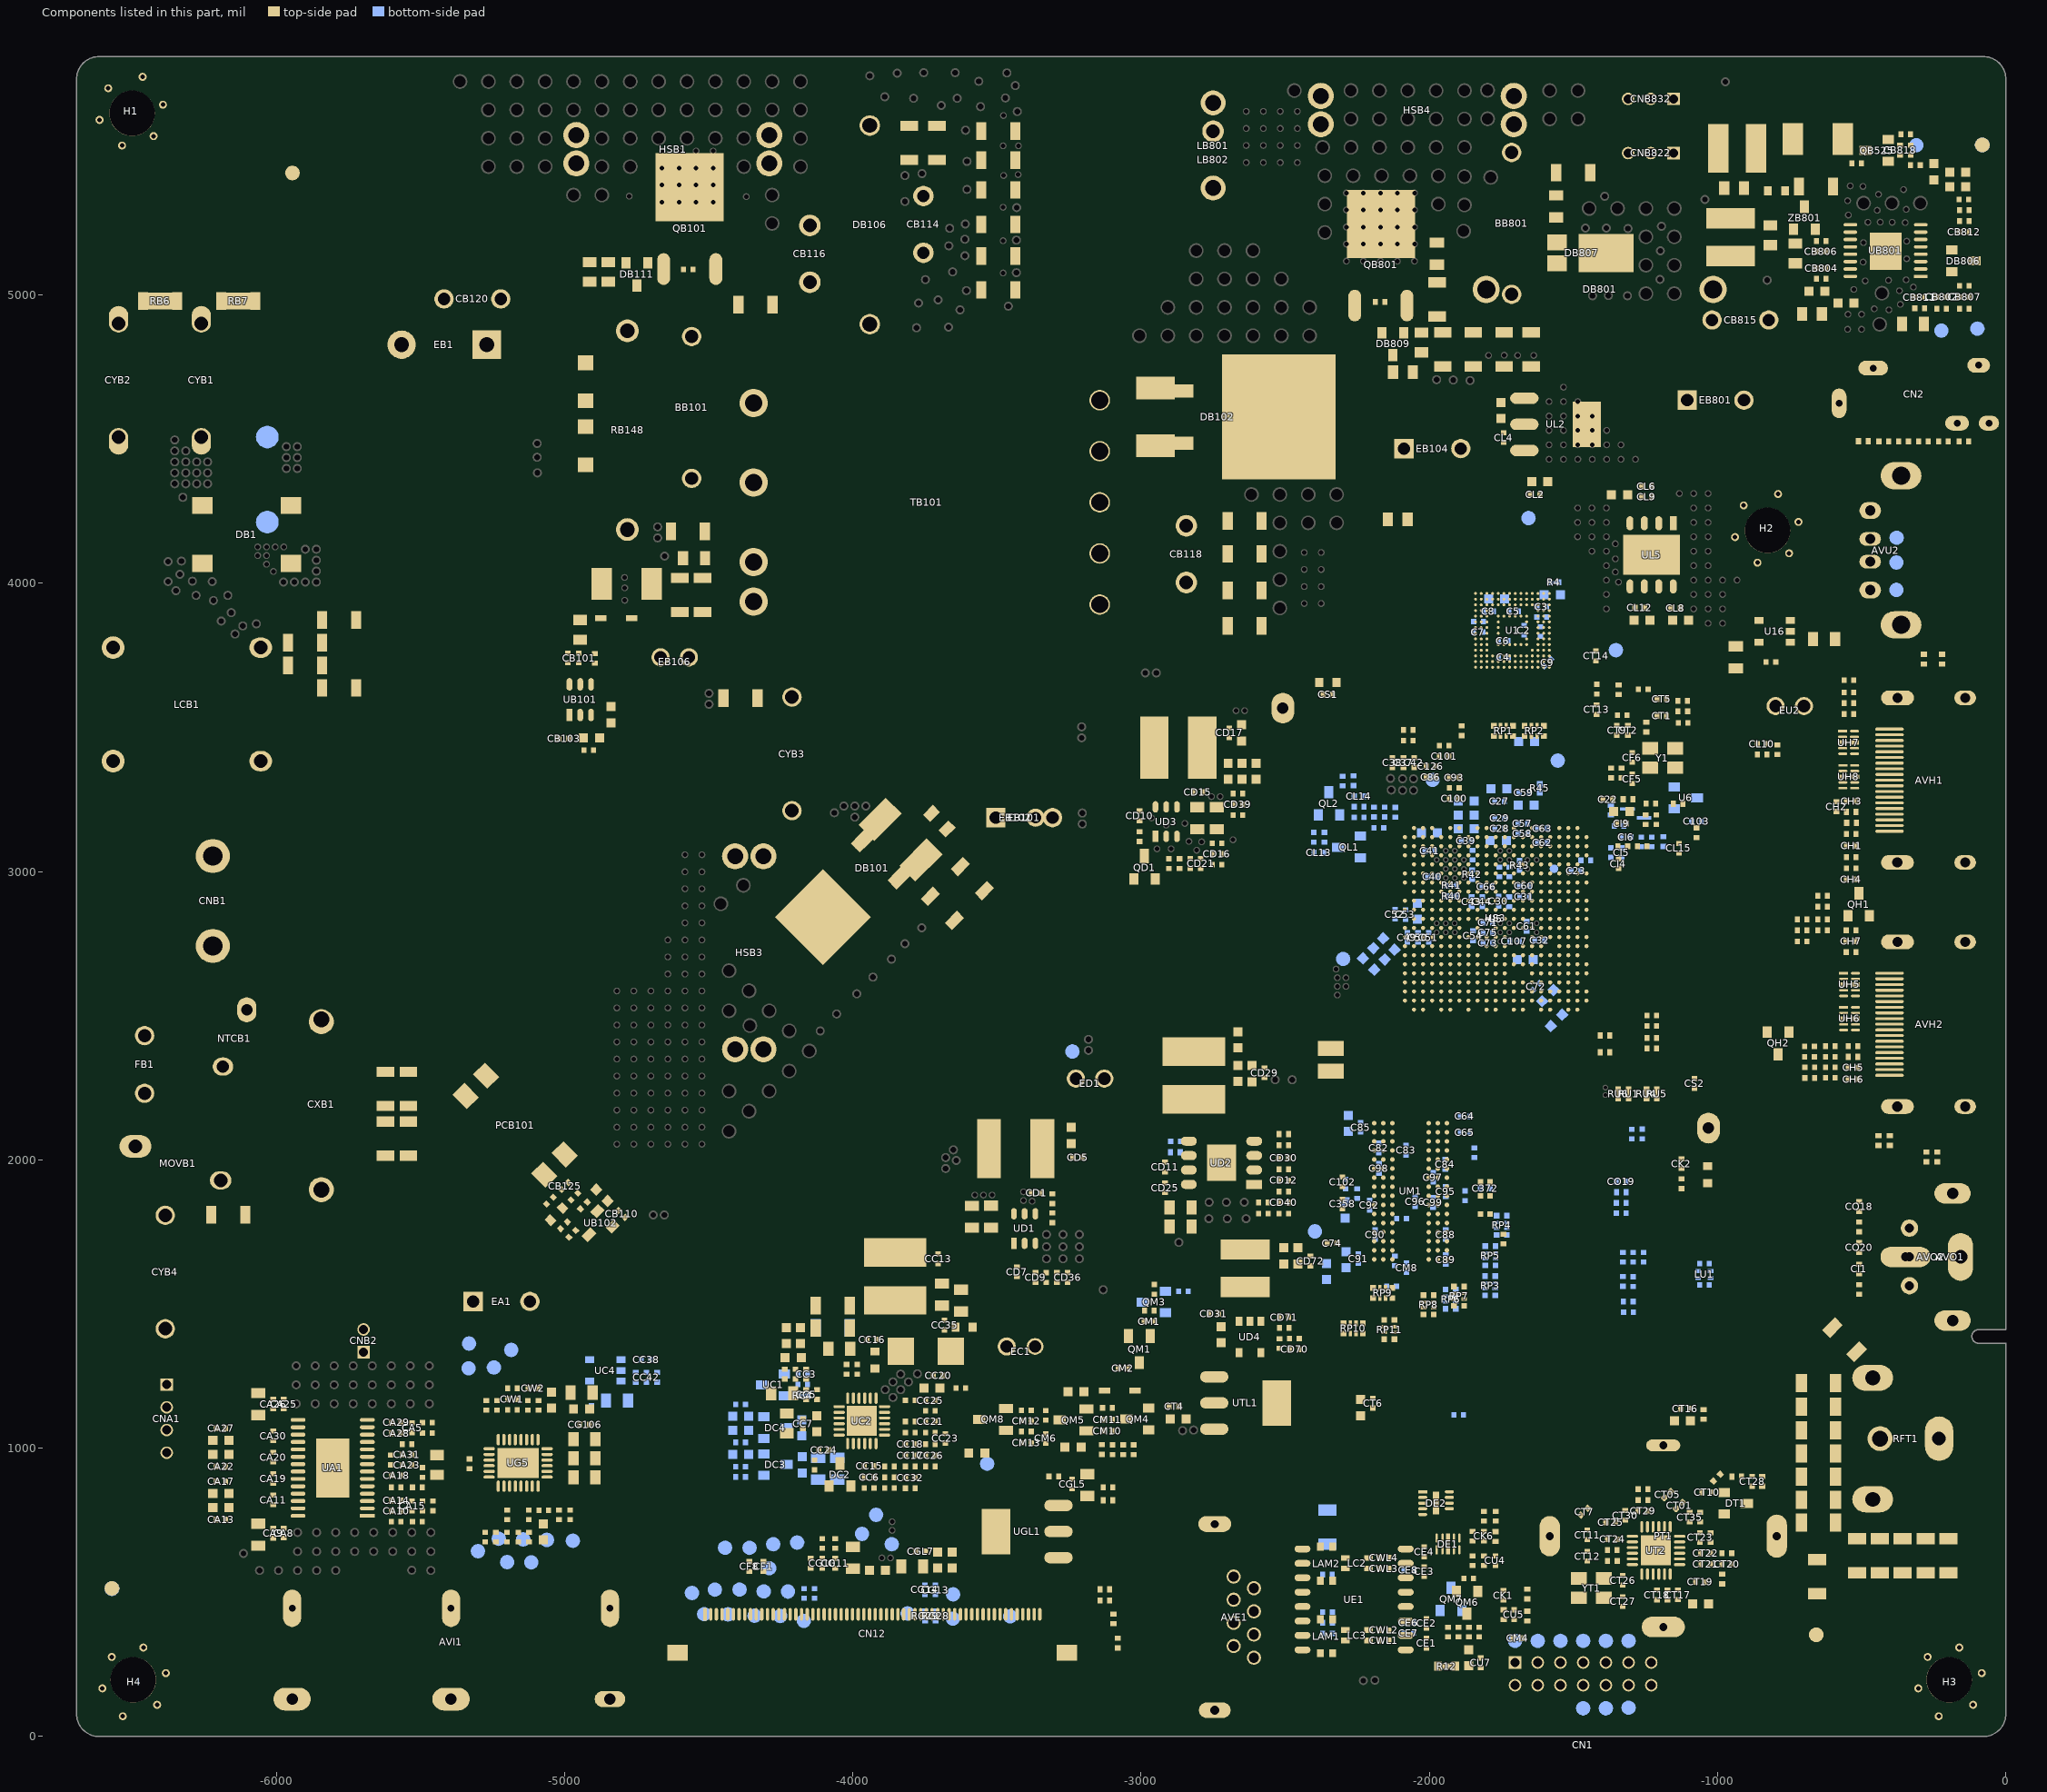
[diagram p0: the components of this part, seen from the top]
# Altium PCB MISC84395.PcbDoc (part 25 of 26)
Units mil, origin at the board's own origin, x right, y up, seen from the top; angles counter-clockwise.
Board outline 6692.91 x 5826.77 mil, 2 copper layers (TopLayer, BottomLayer), stack 61.855 mil thick; 951 components, 565 nets, 4374 pads, 1804 vias.
Unrouted connection lines stored in the file: 1.

## Keep-outs
KeepOutLayer:
  rectangle: 3183.8,-158.59 3314,-79.85
  pour cut-out: -6106,0 -6106,296 -6077,325 -4781.9,325 -4781.9,345 -6088,345 -6132,301 -6132,42 -6174,0
  pour cut-out: -2271,766 -2209,704 -2209,225 -2274,160 -2788,160 -2841,213 -2841,655 -2792,704 -2664.31,704 -2602.31,766
  lines w5: -172,0 -93.26,0 ; 0,118.11 0,590.55 ; 3734.7,-158.59 3734.7,-79.85 ; -6692.91,78.74 ccw(c-6614.17,78.74) -6614.17,0 -78.74,0 ccw(c-78.74,78.74) 0,78.74 0,1364.17 ; -6692.91,78.74 cw(c-6771.65,78.74) -6771.65,0 -13307.09,0 cw(c-13307.09,78.74) -13385.83,78.74 -13385.83,4415.35 -13291.34,4415.35 ccw(c-13291.34,4438.98) -13267.72,4438.98 ccw(c-13291.34,4438.98) -13291.34,4462.6 -13385.83,4462.6 -13385.83,5748.03 cw(c-13307.09,5748.03) -13307.09,5826.77 -6771.65,5826.77 cw(c-6771.65,5748.03) -6692.91,5748.03 ; -6692.91,78.74 -6692.91,5748.03 ; -6692.91,78.74 -6692.91,5748.03 ; -6692.91,5748.03 cw(c-6614.17,5748.03) -6614.17,5826.77 ; -6692.91,5748.03 cw(c-6614.17,5748.03) -6614.17,5826.77 ; -6692.91,5748.03 cw(c-6614.17,5748.03) -6614.17,5826.77 ; -6614.17,5826.77 -78.74,5826.77 ; -78.74,5826.77 cw(c-78.74,5748.03) 0,5748.03 ; -78.74,5826.77 cw(c-78.74,5748.03) 0,5748.03 ; 0,1364.17 -94.49,1364.17 cw(c-94.49,1387.8) -118.11,1387.8 cw(c-94.49,1387.8) -94.49,1411.42 0,1411.42 0,5748.03 ; 0,1364.17 0,1364.17 ; 3183.8,-158.59 3915.83,-158.59 3915.83,-79.85 3183.8,-79.85 3183.8,-158.59
  text "KeepOutLayer" at 3336.6,-137.63 h60
  text ".GKO" at 3758.41,-140.54 h60

## Other copper
TopLayer:
  drawing of 329 lines, arcs and shapes, not listed
  text "TopLayer" at 3349.85,461.03 h60
  text ".GTL" at 3759.34,456.74 h60
BottomLayer:
  drawing of 259 lines, arcs and shapes, not listed
  text ".GBL" at 3759.02,242.51 h60
  text "BottomLayer" at 3336.6,241.01 h60

## Silkscreen, mask and mechanical layers (free items; w line width, h text height)
TopOverlay:
  drawing of 503 lines, arcs and shapes, not listed
  text "LED DRIVER" at -1021.92,5754.78 h60
  text "2" at -7656.83,5661.77 h160 r180
  text "Solder Mask:" at 3048.92,5399.14 h60
  text "IPC SM-840" at 3461.42,5398.14 h60
  text "Silkscreen Color:" at 4227.42,5398.14 h60
  text "White" at 4706.42,5398.14 h60
  text "Units:" at 4227.42,5299.14 h60
  text "PTH Copper Thickness:" at 3048.92,5298.14 h60
  text ">20um" at 3722.42,5297.14 h60
  text "mm" at 4425.42,5297.64 h60
  text "Dielectric Constant Er@1GHz To 1MHz:" at 3048.58,5199.17 h60
  text "4.2 --- 4.6" at 4228.08,5199.67 h60
  text "Panel Size:" at 3046.92,5100.64 h60
  text "2L,2,170.00×148.00mm,FR4(TG130-CTI175),1OZ,Green,OSP,1.6mm" at 3352.08,5100.67 h60
  text "Silkscreen on PTH:" at 3047.42,4999.14 h60
  text "Primary Side Retained;" at 3565.42,4998.14 h60
  text "Secondary Side  Removed for Soldering" at 4227.42,4996.64 h60
  text "Special Requirements" at 3046.41,4908.46 h60
  text "If engineering questions are not answered within 2 hours, please call: PHONE_A" at 4933.08,4901.17 h60
  text "1. Lead-free HASL (HAL_LF, Lead Free Hot Air Leveling)" at 3637.3,4804.87 h60
  text "2. OSP (OSP, Organic Solderability Preservatives)" at 3637.3,4720.87 h60
  text "3. ENIG (ENIG, Electroless Nickel/Immersion Gold)" at 3635.8,4629.37 h60
  text "Plated Technics" at 3121.42,4594.64 h60
  text "4. ENIG + gold finger (ENIG_G/F, Electroless Nickel/Immersion Gold + Gold Finger)" at 3637.3,4548.87 h60
  text "5. Gold plating (Gold_plated, Gold-plated)" at 3638.3,4468.37 h60
  text "6. Gold plating + gold finger (Gold_Plated_G/F, Gold-plated + Gold Finger)" at 3638.8,4390.37 h60
  text "Impedance Control" at 3051.15,4161.78 h60
  text "Target Impedance" at 3847.98,4161.88 h60
  text "Layer(s)" at 5362.12,4161.96 h60
  text "Width & Clearance" at 4593.81,4161.65 h60
  text "75 +/- 10% Ohm" at 3870.18,4061.18 h60
  text "G/12/15.8/12/G mil" at 4551.23,4060.5 h60
  text "layer 1" at 5362.12,4060.62 h60
  text "Single End Impedance" at 3051.15,4014.96 h60
  text "[ Zo ]" at 3274.65,3877.71 h60
  text "G/5/7/5/7/5/G mil" at 4561.23,3669.5 h60
  text "100 +/- 10% Ohm" at 3857.18,3668.49 h60
  text "layer 1" at 5373.11,3666.71 h60
  text "Differential Impedance" at 3051.01,3613.38 h60
  text "[ Zo ]" at 3274.14,3490.05 h60
  text "( G: Ground )" at 3184.22,3382.55 h60
  text "90 +/- 10% Ohm" at 3883.23,3370.5 h60
  text "layer 1&2" at 5369.11,3369.71 h60
  text "G/5/11/5/11/5/G mil" at 4561.23,3367 h60
  text "Common Mode Impedance" at 3030.79,3160.87 h60
  text "[ Zc ]" at 3278.79,3079.87 h60
  text "Refer to Gerber documents GTP&GBP for Stencil aperture design" at 3945.84,2815.68 h60
  text "Stencil" at 3045.08,2718.67 h60
  text "TOP:New" at 3947,2714 h60
  text "BOTTOM:The Same As XXXXXXXXXXXXXXXX XXXXXX" at 3948,2618 h60
  text "Test jig" at 3043.17,2523.02 h60
  text "The Same As XXXXXXXXXXXXXXXX XXXXXX" at 3947.74,2520.12 h60
  text "Wave-soldering jig" at 3045.38,2424.78 h60
  text "The Same As XXXXXXXXXXXXXXXX XXXXXX" at 3951.74,2420.12 h60
  text "Solder paste" at 3943.36,2323 h60
  text "Production process" at 3043.86,2321.5 h60
  text "Note: depanel from the back side" at 4329,2318 h60
  text "This board is 340*148mm, overlength; please pay special attention in production." at 3943.08,2237.17 h60
  text "[Process and notes]" at 3224.08,2236.67 h60
  text "Special requirements" at 3044.86,2123.5 h60
  text "SMD components higher than 2mm on the wave-soldering side" at 3044.58,2022.17 h60
  text "Packaging notes" at 3044.24,1925.95 h60
  text "[Components prone to collision]" at 3285.58,1841.17 h60
  text "Footprint matching" at 3044.24,1725.95 h60
  text "CN1  CN2   AVE1" at 3941.73,1671 h60
  text "[New component footprint]" at 3271.58,1642.17 h60
  text "(Automated Testing Support)" at 3362.58,1527.67 h45
  text "Automatic test support" at 3044.08,1524.17 h60
  text "[Reserved suction cup and press bar positions]" at 3204.58,1439.67 h60
  text "12V" at -5556,1404 h50
  text "GND" at -5557,1318 h50
  text "PWR UPGRADE" at -6244,1312 h60
  text "Layer Stack Up Detail for" at 3185.18,1080.14 h100
  text ".Pcb_File_Name_No_Path" at 4246,1080.14 h100
  text "Layer" at 3349.54,932.41 h50
  text "Gerber" at 3721.26,932.41 h50
  text "Layer" at 4032.4,932.41 h50
  text "Layer" at 4668.64,932.41 h50
  text "Copper" at 5457.54,932.41 h50
  text "Dielectric" at 5769.32,932.41 h50
  text "Stack up" at 4668.64,881.53 h50
  text "Height" at 5769.32,881.53 h50
  text "Name" at 3349.54,880.03 h50
  text "Document" at 3721.26,880.03 h50
  text "Ordor" at 4032.4,880.03 h50
  text "Thickness" at 5457.54,880.03 h50
  text "SPEAKER" at -6666,837 h60
  text "TCON" at -4592,678 h60
  text "TopOverlay" at 3349.24,647.18 h60
  text ".GTO" at 3758.81,644.62 h60
  text "0.4mil" at 5766.64,559.59 h60
  text "1" at 4085.61,456.44 h60
  text "1.4mil" at 5470.6,456.38 h60
  text "2" at 4085.66,243.4 h60
  text "1.4mil" at 5468.89,242.39 h60
  text "1" at -5729,165 h160
  text "0.4mil" at 5769.31,147.71 h60
  text "KEY&IR&LED&EXT-WIFI" at -1082,47 h60
  text "Notes:" at 3021.11,-415.17 h80
  text "1. No Plated Through Hole  overlap each other should be combined ,Residues between them should be eliminated." at 3020.24,-503.08 h60
  text "2. Plated Through Hole superposition should be made as a bigger one." at 3020.18,-579.18 h60
  text "3. When there is not enough space for UL authentication marking,Manufacturer ID code and the Bar Code frame," at 3020.24,-647.68 h60
  text "only the Manufacturer  ID code is needed and layed wherever it can be." at 3078.62,-718.37 h60
  text "4. Spacing between two pads of IC package should be covered with solder oil." at 3020.24,-795.14 h60
  text "5. All trace should be covered with green oil unless otherwise specified. If discovers unusually, please confirm with us." at 3020.24,-868.55 h60
  text "6. Silkscreen overlaped SMD pads should be removed directly." at 3020.24,-941.86 h60
  text "7. The width of Carbon Sprayed must be 16mil wider than its trace." at 3020.24,-1012.9 h60
  text "8. Bridging Thickness of V-cut  should be kept within 0.3±0.1mm when the width of single piece bare board is smaller than 20mm." at 3020.24,-1087.33 h60
  text "9. There is no need to plugged with green oil when the diameter of vias is bigger than 0.6mm." at 3020.24,-1169.16 h60
  text "10. All vias under BGA must be covered and plugged with Solder oil." at 3020.25,-1249.03 h60
BottomOverlay:
  circle w4: c-5607.08,2419.78 r2
  circle w5.91: c-5607.08,2374.41 r2
  circle w4: c-5540.08,2048.78 r2
  circle w5.91: c-5540.08,2003.41 r2
  circle w4: c-5334.08,2419.78 r2
  circle w5.91: c-5334.08,2374.41 r2
  circle w4: c-5342.08,2240.78 r2
  circle w5.91: c-5342.08,2195.41 r2
  circle w4: c-6392.08,2597.78 r2
  circle w5.91: c-6392.08,2552.41 r2
  rectangle: 3183.8,29.07 3314,107.81
  region: 16 vertices and 3 holes, not listed, extent -4142.34,22.62 -3720.14,308.07
  lines w5: -6393.59,2597.76 -6392.08,2566.28 -6390.57,2597.76 ; -5608.59,2419.76 -5607.08,2388.28 -5605.57,2419.76 ; -5541.59,2048.76 -5540.08,2017.28 -5538.57,2048.76 ; -5343.59,2240.76 -5342.08,2209.28 -5340.57,2240.76 ; -5335.59,2419.76 -5334.08,2388.28 -5332.57,2419.76 ; -1348.08,5722.11 -1348.08,5802.23 -1116.22,5802.23 -1116.22,5719.5 ; -1347.98,5456.13 -1347.98,5349 -1116.11,5349 -1116.11,5453.52 ; 3734.7,29.07 3734.7,107.81 ; -6444.91,2540.96 -6342.54,2540.96 -6391.76,2617.73 -6444.91,2540.96 ; -5659.91,2362.96 -5557.54,2362.96 -5606.76,2439.73 -5659.91,2362.96 ; -5592.91,1991.96 -5490.54,1991.96 -5539.76,2068.73 -5592.91,1991.96 ; -5394.91,2183.96 -5292.54,2183.96 -5341.76,2260.73 -5394.91,2183.96 ; -5386.91,2362.96 -5284.54,2362.96 -5333.76,2439.73 -5386.91,2362.96 ; -1163.74,1004 -1163.74,1417.39 -750.35,1417.39 -750.35,1004 -1163.74,1004 ; -542.73,2265.88 -542.73,2679.26 -129.35,2679.26 -129.35,2265.88 -542.73,2265.88 ; -542.73,3112.33 -129.35,3112.33 -129.35,3525.72 -542.73,3525.72 -542.73,3112.33 ; 3183.8,29.07 3183.8,107.81 3915.83,107.81 3915.83,29.07 3183.8,29.07
  lines w6: -6413,1257 -6512,1257 -6512,1183 -6512,949 -6411,949 ; -1224,301 -558,301 -558,24 ; -452,3923 -262,3923 -262,4238 -262,4304 -448,4304 -450,4302
  lines w7.87: -3409,3161 -3409,3217 -3381,3245 -3374,3245 -3292,3245 -3214,3167 -3214,3141 -3214,3126 -3244,3096 -3344,3096 -3402,3154 -3409,3161 ; -2807,5525 -2807,5717 -2792,5732 -2785,5739 -2761,5739 -2708,5739 -2684,5715 -2684,5535 -2715,5504 -2786,5504 -2807,5525
  lines w19.68: -6659.35,1672.8 -6659.35,1477.95 -5881.05,1477.95 -5769,1590 -5567,1590 -4980,2177 -4980,2628 -4827.69,2780.32 -4827.69,2800 -4827.69,3094.19 -4619.87,3302 -4053,3302 -3450,3905 -3450,4518 -3127,4841 -3127,5793 -3323.85,5793 -3323.85,4922.54 -3646.85,4599.54 -3646.85,3986.54 -4134.54,3498.85 -4701.41,3498.85 -5024,3176.26 -5024.54,3175.73 -5024.54,2881.54 -5024.54,2861.85 -5176.85,2709.54 -5176.85,2258.54 -5648.54,1786.85 -5850.54,1786.85 -5962.59,1674.8 -6659.35,1674.8 ; -6667.36,4576.95 -6667.36,4578.95 -6667.36,4773.8 -6285.59,4773.8 -5858.85,5200.54 -5858.85,5781 -5662,5781 -5662,5119 -6204.05,4576.95 -6667.36,4576.95
  text "+" at -1289,5739 h78.74
  text "-" at -1145,5736 h118.11
  text "NC" at -1251.46,5733.63 h50 r270
  text "-" at -1166,5422 h118.11 r180
  text "+" at -1331,5421 h78.74 r180
  text "NC" at -1247,5361 h50 r270
  text "UART" at -318,4603 h60 r270
  text "USB IN" at -79.82,4024.39 h60 r270
  text "HDMI1(ARC) IN(2.0)" at -74.52,3078 h60 r270
  text "FB1" at -6469,2547 h48.31
  text "HDMI2 IN(2.0)" at -74.5,2301 h60 r270
  text "SPDIF OUT" at -478,1554 h50 r270
  text "COAX OUT" at -249,1546 h60 r270
  text "L+" at -6444,1197 h50
  text "RF IN" at -273,1148 h60
  text "L-" at -6448.83,1121 h50
  text "R-" at -6446.27,1045 h50
  text "R+" at -6441.44,971.58 h50
  text "GND" at -1297,365 h50 r270
  text "AV IN" at -5323,251 h60
  text "RJ45 IN" at -2680,201 h60
  text ".GBO" at 3759.43,52.1 h60
  text "BottomOverlay" at 3337.76,51.11 h60
  text "5V_STB" at -865,22 h50 r270
  text "3V3" at -816,22 h50 r270
  text "GND" at -611,22 h50 r270
  text "GND" at -921,21 h50 r270
TopPaste:
  rectangle: 3183.8,722.48 3314,801.22
  lines w5: 3734.7,722.48 3734.7,801.22 ; 3183.8,722.48 3915.83,722.48 3915.83,801.22 3183.8,801.22 3183.8,722.48
  text "TopPaste" at 3349.24,743.71 h60
  text ".GTP" at 3758.81,741.58 h60
BottomPaste:
  rectangle: 3183.8,-65.08 3314,13.66
  lines w5: 3734.7,-65.08 3734.7,13.66 ; 3183.8,-65.08 3915.83,-65.08 3915.83,13.66 3183.8,13.66 3183.8,-65.08
  text "BottomPaste" at 3336.6,-42.1 h60
  text ".GBP" at 3759.7,-47.22 h60
TopSolder:
  rectangle: 3183.8,532.53 3314,611.27
  lines w5: 3734.7,532.53 3734.7,611.27 ; 3183.8,532.53 3915.83,532.53 3915.83,611.27 3183.8,611.27 3183.8,532.53
  text "TopSolder" at 3349.74,552.63 h60
  text ".GTS" at 3758.81,550.98 h60
BottomSolder:
  drawing of 57 lines, arcs and shapes, not listed
  text "BottomSolder" at 3336.6,144.31 h60
  text ".GBS" at 3758.78,143.42 h60
过炉治具:
  drawing of 418 lines, arcs and shapes, not listed
3D和装配:
  lines w5: -6732.29,118.11 -6732.29,0 -6614.18,0 ; -1222.79,944.94 -1222.79,1476.44 -691.3,1476.44 -691.3,944.94 -1222.79,944.94 ; -602.06,2206.94 -602.06,2738.44 -70.56,2738.44 -70.56,2206.94 -602.06,2206.94 ; -601.79,2206.82 -601.79,2738.32 -70.29,2738.32 -70.29,2206.82 -601.79,2206.82 ; -601.79,3053.28 -70.29,3053.28 -70.29,3584.77 -601.79,3584.77 -601.79,3053.28
  lines w70.87: -651,1243 -651,1285 -523,1413 -491,1413 -445,1367 -425,1347 21,1347 ; -651,1268 -651,697 -677,671 -705,671 -715,661 -724,652 -724,600 -724,577 -701,554 -632,554 -604,554 -586,572 -586,603 ; -585,604 -562,627 13,627
  lines w78.74: -2757,631 -2865,631 -2894,602 -2894,266 -2832,204 -2330,204 -2248,286 -2248,684 -2290,726 -2542,726
  text "2L,2,170.00×148.00mm,FR4(TG130-CTI175),1OZ,Green,OSP,1.6mm,6,48,88.8%,3040,0.3mm" at 3352.08,5100.67 h60
自动测试:
  circle w6: c-3794.77,3473.17 r196.85
  circle w6: c-3793.64,3473.17 r236.22
  circle w6: c-3143.64,5078.17 r236.22
  circle w6: c-3144.77,5078.17 r196.85
  circle w6: c-5956.64,5561.17 r236.22
  circle w6: c-5957.77,5561.17 r196.85
  circle w6: c-5802.64,5090.17 r236.22
  circle w6: c-5803.77,5090.17 r196.85
  circle w6: c-4777.64,3153.17 r236.22
  circle w6: c-4778.77,3153.17 r196.85
  circle w6: c-4799.64,2329.17 r236.22
  circle w6: c-4800.77,2329.17 r196.85
  circle w6: c-5444.64,2628.17 r236.22
  circle w6: c-5445.77,2628.17 r196.85
  circle w6: c-1867.48,1138.73 r196.85
  circle w6: c-1866.35,1138.73 r236.22
  circle w6: c-877.27,1524.17 r196.85
  circle w6: c-876.14,1524.17 r236.22
  circle w6: c-2960.77,2700.67 r196.85
  circle w6: c-2959.64,2700.67 r236.22
  circle w6: c-3763.77,2362.17 r196.85
  circle w6: c-3762.64,2362.17 r236.22
  circle w6: c-4525.77,892.17 r196.85
  circle w6: c-4524.64,892.17 r236.22
顶层限制:
  drawing of 5211 lines, arcs and shapes, not listed
  text "Height limit 8mm" at -4175.97,8015.84 h201.68
  text "165.1" at -3414.04,6709.3 h98.43
  text "160.15" at -3357.61,6474.12 h98.43
  text "31.25" at -795.6,6237.9 h98.43
  text "21" at -479,6001.68 h98.43
  text "A" at -6710.04,5888.16 h201.68
  text "2" at -1303.15,5569.69 h31.5 r180
  text "1" at -1145.67,5569.69 h31.5 r180
  text "B" at -6152.98,5422.13 h201.68
  text "LED DRIVER" at -1705.68,5226.98 h118.11
  text "6-22054" at -5684.66,5093.37 h98.43
  text "5" at 3417.61,4831.85 h78.74 r90
  text "L" at -6228.5,4712.53 h78.74 r270
  text "L" at -6178.05,4712.53 h78.74 r90
  text "6" at 3553.44,4624.17 h78.74 r90
  text "UART" at 4297.26,4513.08 h201.68
  text "2.5" at 4091.82,4498.19 h78.74 r180
  text "0.5" at 4175.52,4396.33 h98.43 r180
  text "AC IN" at -6171.77,4376.58 h50 r270
  text "AC IN" at -6141.77,4376.58 h50 r90
  text "GND" at -229.37,4245.34 h50
  text "A" at -1162.97,4223.7 h201.68
  text "DP" at -228.37,4138.34 h50
  text "N" at -6230.05,4125.82 h78.74 r270
  text "N" at -6179.61,4125.82 h78.74 r90
  text "DM" at -228.37,4059.34 h50
  text "5V" at -228.37,3990.34 h50
  text "14.4" at 3416.66,3967.72 h98.43 r90
  text "USB" at 4297.26,3937.01 h201.68
  text "7.0" at 4178.26,3934.22 h98.43 r180
  text "0.55" at 4240.96,3613.62 h98.43 r180
  text "AC IN" at -6558.88,3604.93 h201.68
  text "15" at 3483.46,3243.01 h98.43 r90
  text "HDMI1(ARC)" at 4297.26,3176.5 h201.68
  text "L" at -6228.5,3173.36 h78.74 r270
  text "L" at -6178.05,3173.36 h78.74 r90
  text "6.1" at 4129.58,3105.59 h98.43 r180
  text "AC IN" at -6171.77,2837.41 h50 r270
  text "AC IN" at -6141.77,2837.41 h50 r90
  text "148" at 2347.49,2798.56 h98.43 r90
  text "0.55" at 4240.96,2767.16 h98.43 r180
  text "143" at -7966.53,2700.13 h98.43 r90
  text "N" at -6230.05,2586.65 h78.74 r270
  text "N" at -6179.61,2586.65 h78.74 r90
  text "138.05" at -7730.31,2496.06 h98.43 r90
  text "15" at 3483.46,2396.55 h98.43 r90
  text "HDMI2" at 4297.26,2262 h201.68
  text "6.1" at 4129.58,2259.13 h98.43 r180
  text "118.25" at 2111.27,2114.55 h98.43 r90
  text "Top and bottom keep-out" at 43.93,2032.24 h59.06
  text "8.5" at 3603.04,2003.39 h98.43 r180
  text "Components and traces" at 43.93,1923.97 h59.06
  text "104.5" at 1638.82,1884.9 h98.43 r90
  text "106.25" at 1875.04,1870.08 h98.43 r90
  text "8.3" at 3271.23,1777.17 h78.74 r146
  text "1.9" at 3908.04,1712.39 h98.43 r180
  text "6.5" at 3960.99,1668.31 h78.74 r90
  text "9.5" at 3298.04,1597.39 h98.43 r90
  text "11.5" at 3241.51,1533.47 h78.74 r180
  text "6" at 3881.04,1488.39 h98.43 r180
  text "84.25" at 1402.6,1461.61 h98.43 r90
  text "COAX & optical fiber" at 4299.53,1432.64 h201.68
  text "11.4" at 3642.04,1362.39 h98.43 r180
  text "SPK" at -6421.57,1345.41 h201.68
  text "73.51" at -7494.09,1266.68 h98.43 r90
  text "1" at -6535.44,1228.35 h31.5 r270
  text "6.3" at 3857.16,1179.13 h78.74
  text "2" at -6535.44,1153.54 h31.5 r270
  text "3" at -6535.44,1078.74 h31.5 r270
  text "62.75" at 1166.38,1038.39 h98.43 r90
  text "4" at -6535.44,1000 h31.5 r270
  text "1" at -257.22,925.17 h98.43
  text "RF" at 4297.26,923.76 h201.68
  text "11.2" at 3225.27,902.56 h78.74 r90
  text "ÂÌÉ«ÄÚÈ¦ÊÇÊµ¼ÊÏÂ³ÁÇøÓò£¬Ô¤Áô5mm²È«¾àÀë£¬ÏÞ¸?.5mm" at -6222.28,837.42 h118.11
  text "42.25" at 930.16,634.87 h98.43 r90
  text "Top and bottom keep-out" at 59.21,596.39 h59.06
  text "TCON" at -4178.35,572.25 h118.11
  text "Components and traces" at 59.21,488.12 h59.06
  text "28" at -7257.87,469.16 h98.43 r90
  text "8.5" at -7426.68,383.86 h98.43
  text "B" at -673,383.97 h201.68
  text "A" at -6414.77,379.86 h201.68
  text "KEY&WIFI" at -1533.88,348.88 h118.11
  text "26.25" at 699.21,319.88 h98.43 r90
  text "15.7" at 3265.64,289.23 h78.74 r90
  text "2.25" at -1172.51,147.64 h98.43
  text "10" at 462.99,139.44 h98.43 r90
  text "10.95" at -2226.77,131.69 h78.74 r180
  text "13.0" at 3159.34,127.81 h78.74 r180
  text "5" at -6818.41,65.62 h98.43 r90
  text "5" at 226.77,65.62 h98.43 r90
  text "A" at -605.71,58.37 h201.68
  text "10.52" at -2103.44,34.87 h98.43 r90
  text "5" at -131.23,-219.11 h98.43
  text "5.25" at -4534.04,-246.06 h98.43
  text "4.5" at -2119.75,-246.06 h98.43
  text "9.95" at -343.5,-455.33 h98.43
  text "L IN" at -5141.78,-660.11 h201.68 r90
  text "R IN" at -4716.23,-662.19 h201.68 r90
  text "RJ45" at -2909.17,-662.19 h201.68 r90
  text "31.25" at -795.6,-691.55 h98.43
  text "37.25" at -930.12,-927.78 h98.43
  text "CVBS IN" at -5881.11,-1094.14 h201.68 r90
  text "71.21" at -1565.82,-1164 h98.43
  text "100" at -2066.93,-1400.22 h98.43
  text "137" at -2811.68,-1636.44 h98.43
  text "165" at -3362.86,-1872.66 h98.43
  text "170" at -3453.09,-2108.88 h98.43
  text "3- 8.3" at -6151.71,-2540.65 h98.43
  text "0.43" at -4306.1,-2660.1 h98.43
  text "14" at -5209.78,-2729.91 h98.43
  text "14" at -5746.78,-2745.91 h98.43
  text "11" at -2852.77,-2908.39 h98.43
  text "5.1" at -4244.99,-3007.1 h98.43
  text "13" at -2288.09,-3319.22 h98.43 r90
  text "1.6" at -22.07,-3361.87 h98.43
  text "35.13" at -4117.76,-3819.89 h98.43
  text "9.6" at -5194.78,-3946.91 h98.43 r90
  text "19.3" at -4764.77,-3973.91 h98.43 r90
底层限制:
  circle w5: c-6500,5629.92 r78.74
  circle w5: c-6305.12,5435.04 r78.74
  circle w5: c-391.73,393.7 r236.22
  circle w5: c683.28,4521.66 r118.11
  circle w5: c-8379.26,5433.07 r885.83
  circle w5: c-8379.26,5433.07 r649.61
  circle w5: c-826.77,4183.07 r393.7
  circle w5: c-6496.07,196.85 r393.7
  circle w5: c-6496.07,196.85 r78.74
  circle w5: c-196.85,196.85 r78.74
  circle w5: c-826.77,4183.07 r78.74
  circle w5: c-391.73,393.7 r78.74
  lines w5: -9329.15,6101.26 -9280.84,6187.01 ; -9275.41,6296.92 -8715.66,5981.57 ; -9224.12,6287.68 -9232.53,6272.77 ; -9126.49,5433.07 -6299.22,5433.07 ; -9078.56,6646.33 -8518.81,6330.98 ; -9044.08,6607.26 -9035.68,6622.17 ; -8987.37,6707.93 -8939.06,6793.68 ; -8792.64,4591.25 -8792.64,6043.31 ; -8792.64,7469.29 -8792.64,6043.31 ; -8595.79,4511.38 -8595.79,5895.67 -8792.64,6043.31 ; -8595.79,5781.43 -8379.26,5599.73 ; -8497.37,6318.9 -8379.26,6318.9 ; -8379.26,5071.55 -8379.26,5599.73 ; -8379.26,5505.91 -8300.52,5505.91 -8300.52,5360.24 ; -8379.26,7574.01 -8379.26,5599.73 ; -6692.92,4547.25 -6299.22,4547.25 ccw(c-6299.22,5433.07) -5413.39,5433.07 -5413.39,5826.77 ; -6692.92,4783.47 -6299.22,4783.47 ccw(c-6299.22,5433.07) -5649.61,5433.07 -5649.61,5826.77 ; -1786.21,3611.33 -1046.3,4115.81 ; -1018.11,687.95 -919.68,687.95 -684.04,556.62 ; -826.77,4183.07 1460.18,4183.07 ; -99.42,230.78 -13.45,182.87 ; 683.28,3245.04 683.28,5013.24 ; 683.28,4128.94 781.71,4128.94 ; 683.28,4237.21 781.71,4237.21 ; 683.28,4521.66 801.39,4521.66 ; 702.97,4109.25 781.71,4109.25 ; 702.97,4256.89 781.71,4256.89 ; 781.71,4109.36 781.71,4256.79 ; 899.82,3834.72 683.28,4016.41 683.28,4349.73 899.82,4531.43 ; 919.5,3843.9 702.97,4025.59 702.97,4340.55 919.5,4522.25 ; -9232.53,6272.77 -9295.13,6195.06 -9266.55,6178.96 -9232.53,6272.77 ; -9035.68,6622.17 -8973.08,6699.88 -9001.66,6715.98 -9035.68,6622.17 ; -6692.92,78.74 ccw(c-6614.18,78.74) -6614.18,0 -78.74,0 ccw(c-78.74,78.74) 0,78.74 0,1364.17 -94.49,1364.17 cw(c-94.49,1387.8) -118.11,1387.8 cw(c-94.49,1387.8) -94.49,1411.42 0,1411.42 0,5748.03 ccw(c-78.74,5748.03) -78.74,5826.77 -6614.18,5826.77 ccw(c-6614.18,5748.03) -6692.92,5748.03 ; -6692.92,78.74 -6692.92,5748.03 ; -6692.92,78.74 -6692.92,5748.03 ; -598.07,508.7 -676.06,570.95 -692.03,542.29 -598.07,508.7 ; -598.07,508.7 -185.4,278.7 ; -185.4,278.7 -107.41,216.45 -91.44,245.11 -185.4,278.7 ; -6773.29,5350.37 cw(c-6496.07,5629.92) -6217.56,5908.19 -6027.71,5718.18 cw(c-6299.22,5433.07) -6577.61,5154.69 -6773.29,5350.37 ; -668.95,114.15 cw(c-391.73,393.7) -113.22,671.97 76.62,481.96 cw(c-194.88,196.85) -473.27,-81.53 -668.95,114.15
  text "10.19" at -9014.74,6559.09 h98.43 r60.6
  text "USB solder pins enter this area," at -1837.15,3469.91 h157.48
  text "Acceptable to customer" at -1838.92,3177.36 h157.48
  text "220512" at -1045.67,638.74 h98.43